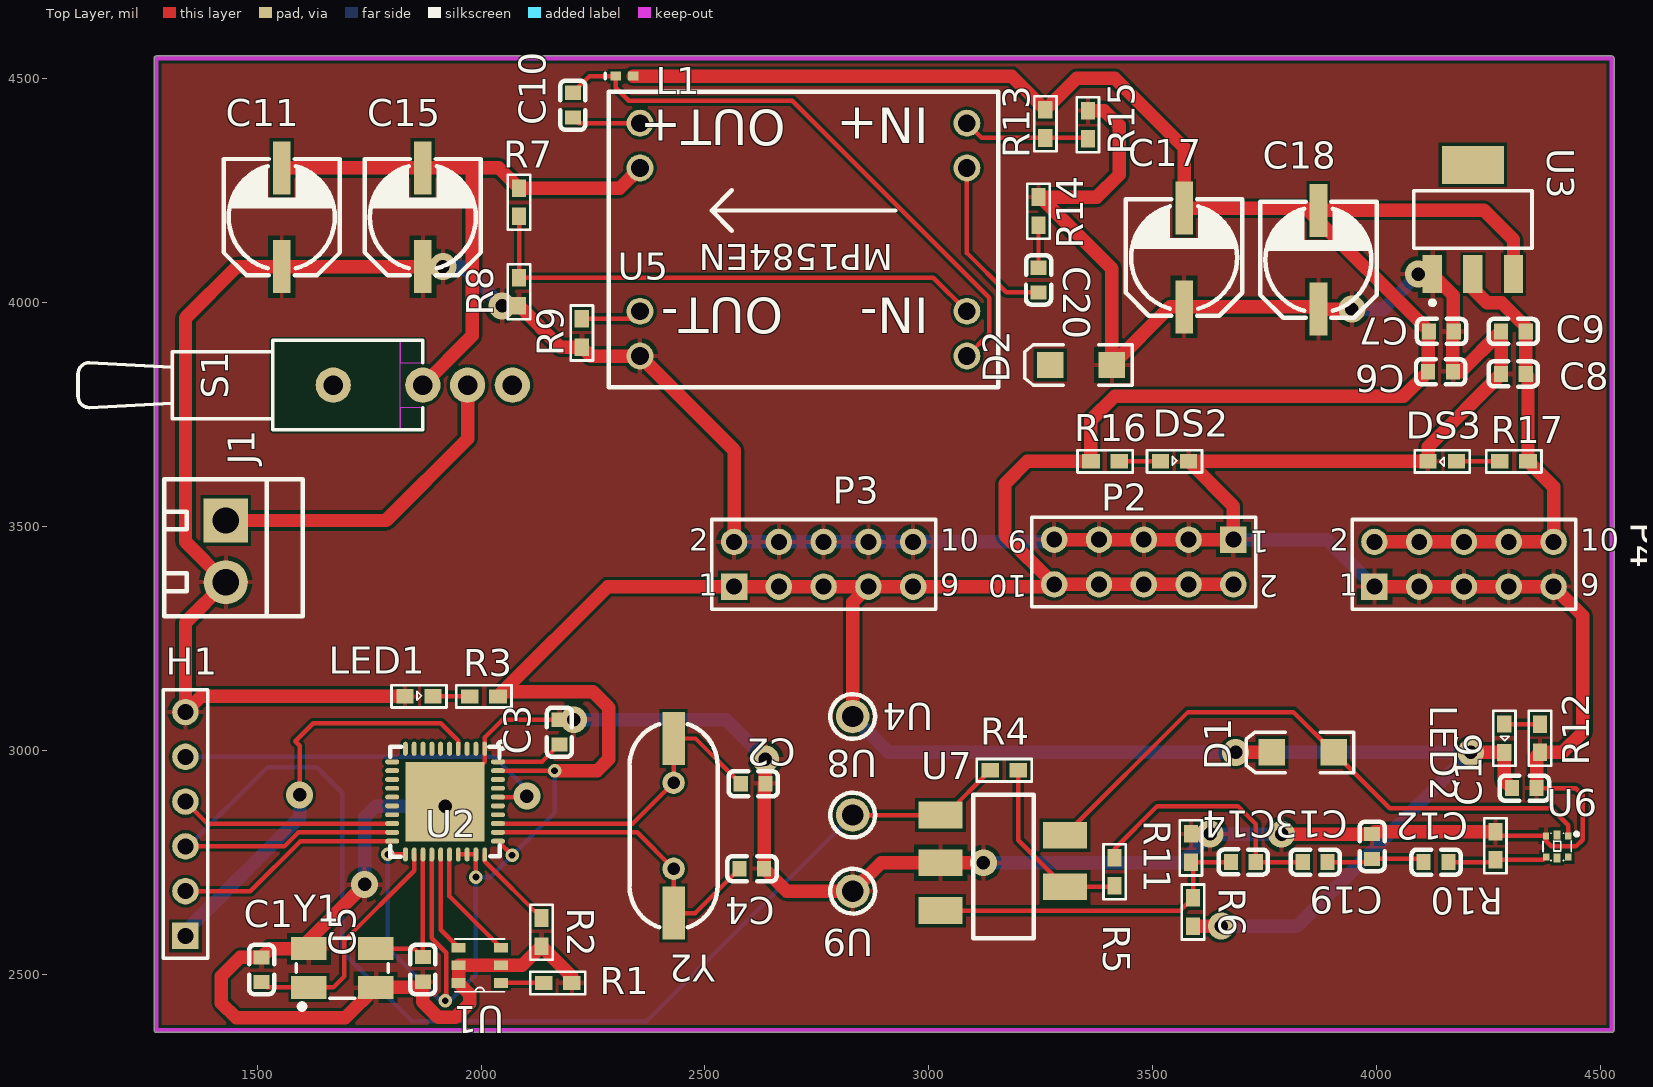
[diagram p0: Top Layer view]
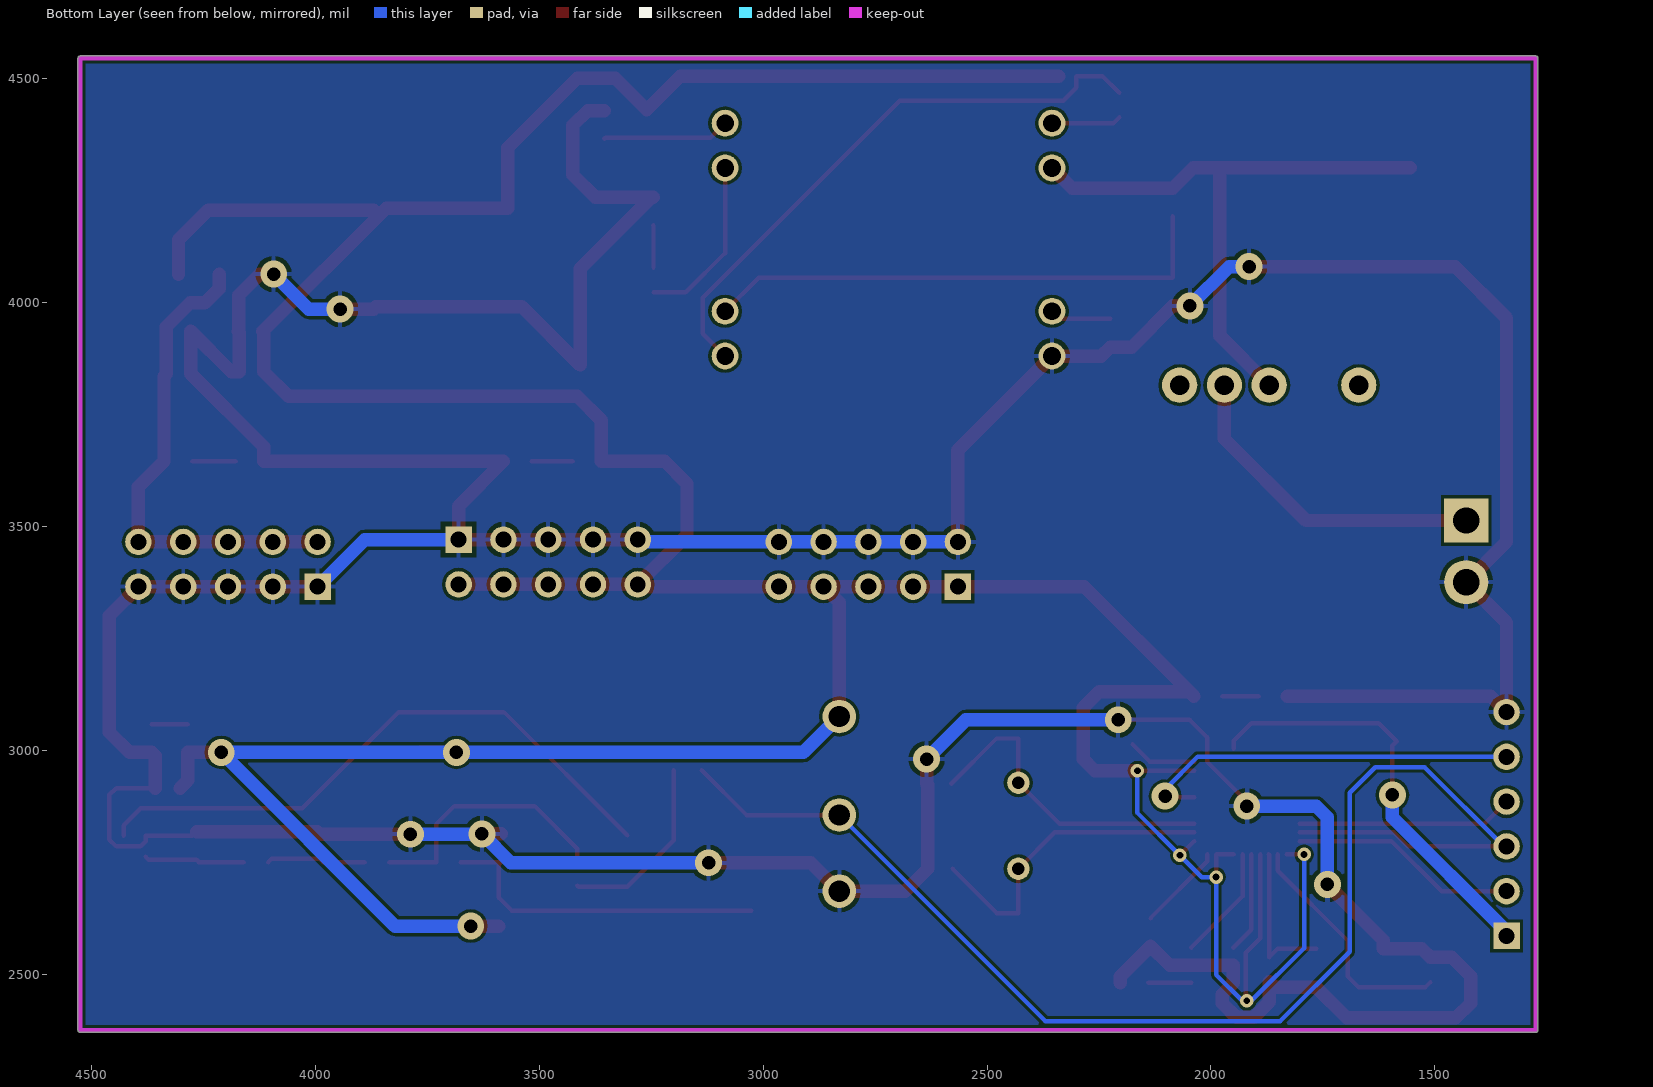
[diagram p1: Bottom Layer view, seen from below]
# Altium PCB MISC80555.PcbDoc
Units mil, origin at the board's own origin, x right, y up, seen from the top; angles counter-clockwise.
Board outline 3260.03 x 2180.03 mil, 2 copper layers (Top Layer, Bottom Layer); 61 components, 36 nets, 211 pads, 21 vias.

## Layer stack, top to bottom (the 12.6 mil dielectric is the usual default, probably not edited)
Top Solder: solder mask 0.4, Solder Resist, Dk 3.5
Top Layer: signal copper 1.4
Dielectric 1: dielectric 12.6, FR-4, Dk 4.8
Bottom Layer: signal copper 1.4
Bottom Solder: solder mask 0.4, Solder Resist, Dk 3.5

## Board outline
1275,2369.99 cw(c1275,2375) 1269.98,2375 1269.98,4545 cw(c1275,4545) 1275,4550.02 4525,4550.02 cw(c4525,4545) 4530.02,4545 4530.02,2375 cw(c4525,2375) 4525,2369.99

## Design rules (kind name [scope] priority, off if disabled: settings)
Clearance [All] p1: gap=7 ignorepadtopadclearanceinfootprint=FALSE except(0: Arc-Hole Track-Hole SMDPad-Hole THPad-Hole Via-Hole Fill-Hole Poly-Hole Region-Hole Text-Hole)
MinimumSolderMaskSliver [All] p1: minsoldermaskwidth=0
PolygonConnect [All] p1: connectstyle=Relief reliefconductorwidth=10 reliefentries=4 polygonreliefangle="90 Angle" airgapwidth=10
RoutingVias [All] p1: holewidth=28 width=50 viastyle="Through Hole" minholewidth=28 minwidth=50 maxholewidth=28 maxwidth=50
SilkToSilkClearance [All] p1: silktosilkclearance=0
SilkToSolderMaskClearance [IsPad] p1: minsilkscreentomaskgap=0 clearancetoexposedcopper=TRUE
SolderMaskExpansion [All] p1: expansion=4
Width [All] p1: maxlimit=30 minlimit=10 preferedwidth=10
27 further rules are at their usual default settings.

## Components (designator, comment, footprint, x,y, rotation, side; value= is the part's Value field where it differs from the comment)
C1 "100nF" C0603 1510,2510 r270 top
C2 "100nF" C0603 2607.75,2924.89 r180 top
C3 "100nF" C0603 2175,3040 r90 top
C4 "100nF" C0603 2605,2735 r180 top
C5 "100nF" C0603 1870,2510 r90 top
C6 "100nF" C0603 4142.86,3844.89 r180 top
C7 "100nF" C0603 4145,3935 r180 top
C8 "100nF" C0603 4305,3840 r0 top
C9 "100nF" C0603 4305,3935 r0 top
C10 "100nF" C0603 2205,4440 r90 top
C11 "220UF/25V" 贴片电容 1555,4190 r0 top
C12 "100nF" C0603 4132.75,2749.89 r180 top
C13 "100nF" C0603 3862.86,2749.89 r180 top
C14 "100nF" C0603 3702.25,2750.11 r0 top
C15 "10UF/50V" 贴片电容 1870,4190 r0 top
C16 "100nF" C0603 4330,2915 r180 top
C17 "22UF/50V" 贴片电容 3570,4100 r0 top
C18 "220UF/25V" 贴片电容 3870,4095 r0 top
C19 "100nF" C0603 3990,2785 r270 top
C20 "100nF" C0603 3245,4050 r270 top
D1 "D_1N4007A" 3.2X1.6X1.1 3835,2995 r180 top
D2 "Diode BAS16" 3.2X1.6X1.1 3340,3860 r180 top
DS2 "LED2" my0603LED 3517.01,3645 r0 top
DS3 "LED2" my0603LED 4177.99,3645 r180 top
H1 "HDR-F_2.54_1x6P" HDR1X6 1340,2585 r90 top
J1 "KF350-2P" KF350-2P 1430,3512.8 r270 top
L1 "10UH" 0402-A 2320.31,4505 r0 top
LED1 "LED_0603-R" my0603LED 1830,3120.24 r0 top
LED2 "LED_0603-R" my0603LED 4285,3057.99 r270 top
P2 "Header 5X2" HDR2X5 3680,3470 r180 top
P3 "Header 5X2" HDR2X5 2565,3365 r0 top
P4 "Header 5X2" HDR2X5 3995,3365 r0 top
R1 "10K" my0603 2140,2480 r0 top
R2 "10K" my0603 2135,2625 r270 top
R3 "10K" my0603 2037.99,3120 r180 top
R4 "10K" my0603 3137.01,2955 r0 top
R5 "10K" my0603 3415,2760 r270 top
R6 "10K" my0603 3590,2670 r270 top
R7 "10K" my0603 2085,4192.01 r90 top
R8 "10K" my0603 2085,3992.01 r90 top
R9 "10K" my0603 2225,3900 r90 top
R10 "10K" my0603 4265,2817.99 r270 top
R11 "10K" my0603 3585,2812.99 r270 top
R12 "10K" my0603 4365,2995 r90 top
R13 "10K" my0603 3260,4430 r270 top
R14 "10K" my0603 3245,4172.01 r90 top
R15 "10K" my0603 3355,4365 r90 top
R16 "10K" my0603 3425,3645 r180 top
R17 "10K" my0603 4337.99,3645 r180 top
S1 "SW-SPDT" TL36WW15050 1870,3815 r180 top
U1 "BL1" "TSOP-6 - duplicate" 1997.24,2519.37 r180 top
U2 "CC2540" CC254X_QFN 1920,2885 r270 top
U3 "LM1117-3.3" LM1117-3.3 4205,4175 r270 top
U4 "RH-5000" TEST-TH_BD2.54-P1.4_RED 2830,3075 r180 top
U5 "MP1584EN" MP1548EN 2720,4140 r180 top
U6 "APDS" SENSORS-SMD_APDS-9008-020 4410,2785 r0 top
U7 "AMP" MCP6001 3165,2740 r0 top
U8 "RH-5000" TEST-TH_BD2.54-P1.4_RED 2830,2855 r180 top
U9 "RH-5000" TEST-TH_BD2.54-P1.4_RED 2830,2685 r180 top
Y1 "12MHz" OSC-SMD_4P-L5.0-W3.2-BL 1690.2,2502.82 r0 top
Y2 "8MHz" XTAL_US 2430,2927.13 r270 top

## Footprints (in the part's own frame and the unit in brackets; to place one, negate y for a bottom-side part, rotate by r counter-clockwise, add the part's x,y. Pads: shape width x height; smd on the part's side, far side on the other; paste and mask are expansions set on the pad)
3.2X1.6X1.1 [mm] "SMT LED; 2 Flat Leads"
  rect 1.5x1.5 smd: 1(-1.75,0) 2(1.75,0)
  silkscreen extent -2.9,-1.15 3.2,1.15
0402-A [mm] "Chip Inductor, Body 1.0x0.5mm, IPC High Density"
  rect 0.6x0.5 smd: 1(-0.5,0) 2(0.5,0)
  silkscreen extent -1.1,-0.15 -1.1,0.15, body extent -0.55,-0.3 0.55,0.3, height 0.55
C0603 [mm]
  rect 0.8x0.9 smd paste+0 mask+0.051: 1(-0.692,-0.003) 2(0.708,-0.003)
  silkscreen extent -1.4,-0.71 1.4,0.71
CC254X_QFN [mm]
  oval 0.8x0.28 smd paste+0 mask+0.051: 1(-2.998,2.242) 2(-2.998,1.742) 3(-2.998,1.242) 4(-2.998,0.742) 5(-2.998,0.242) 6(-2.998,-0.258) 7(-2.998,-0.758) 8(-2.998,-1.258) 9(-2.998,-1.758) 10(-2.998,-2.258) 21(2.996,-2.254) 22(2.998,-1.758) 23(2.998,-1.258) 24(2.998,-0.758) 25(2.998,-0.258) 26(2.998,0.242) 27(2.998,0.742) 28(2.998,1.242) 29(2.998,1.742) 30(2.998,2.242)
  oval 0.28x0.8 smd paste+0 mask+0.051: 11(-2.256,-3.007) 12(-1.756,-3.007) 13(-1.256,-3.007) 14(-0.756,-3.007) 15(-0.256,-3.007) 16(0.244,-3.007) 17(0.744,-3.007) 18(1.244,-3.007) 19(1.744,-3.007) 20(2.244,-3.007) 31(2.244,2.99) 32(1.744,2.99) 33(1.244,2.99) 34(0.744,2.99) 35(0.244,2.99) 36(-0.256,2.99) 37(-0.756,2.99) 38(-1.256,2.99) 39(-1.756,2.99) 40(-2.256,2.99)
  rect 4.5x4.5 smd paste+0 mask+0.051: 41(0,-0.008)
  silkscreen extent -3.4,-3.12 3.12,3.41
HDR1X6 [mm] "Connector; Header; 6 Position"
  rect 1.5x1.5 hole 0.9: 1(0,0)
  round 1.5 hole 0.9: 2(2.54,0) 3(5.08,0) 4(7.62,0) 5(10.16,0) 6(12.7,0)
  silkscreen extent -1.27,-1.27 13.97,1.27
HDR2X5 [mm] "Connector; Header; 5x2 Position"
  rect 1.5x1.5 hole 0.9: 1(0,0)
  round 1.5 hole 0.9: 2(0,2.54) 3(2.54,0) 4(2.54,2.54) 5(5.08,0) 6(5.08,2.54) 7(7.62,0) 8(7.62,2.54) 9(10.16,0) 10(10.16,2.54)
  silkscreen extent -1.27,-1.27 11.43,3.81
KF350-2P [mm] "可拼接端子/10A"
  rect 2.5x2.5 hole 1.5: 1(0,0)
  round 2.5 hole 1.5: 2(3.5,0)
  silkscreen extent -2.34,-3.48 5.44,4.37, body extent -2.15,-3.34 5.25,4.16, height 10
LM1117-3.3 [mm]
  rect 2.15x1.1 smd: 1(2.846,-2.046) 2(2.846,0.254) 3(2.846,2.554)
  rect 2.15x3.5 smd: 4(-3.354,0.254)
  silkscreen extent -1.88,-3.1 4.6,3.6
MCP6001 [mil]
  rect 98.42x60 smd paste+4 mask+4: 1(-138.75,115) 2(-138.75,8.33) 3(-138.75,-98.33) 4(138.75,-45) 5(138.75,70)
  silkscreen extent -66,-160 69,160
MP1548EN [mil]
  round 60 hole 39.37 paste+4 mask+4: 1(-365.04,260) 2(-365.04,160) 3(-365.04,-160) 4(-365.04,-260) 5(364.96,260) 6(364.96,160) 7(364.96,-160) 8(364.96,-260)
  silkscreen extent -435,-330 435,330
my0603 [mm]
  rect 1x0.8 smd: 1(0,0) 2(1.6,0)
  silkscreen extent -0.76,-0.64 2.36,0.64
my0603LED [mm]
  rect 0.965x0.8 smd: 1(0,0) 2(1.6,0)
  silkscreen extent -0.76,-0.64 2.36,0.64
OSC-SMD_4P-L5.0-W3.2-BL [mm]
  rect 2x1.3 smd paste+0 mask+0.102: 1(-1.9,-0.834) 2(1.9,-0.834) 3(1.9,1.366) 4(-1.9,1.366)
  silkscreen extent -2.6,-2.07 2.6,1.97
SENSORS-SMD_APDS-9008-020 [mm]
  rect 0.35x0.4 smd paste+0 mask+0.051: 1(0.45,0.596) 3(-0.8,0.596) 4(-0.799,-0.6) 6(0.451,-0.6)
  rect 0.4x0.5 smd paste+0 mask+0.051: 2(-0.173,0.65) 5(-0.173,-0.65)
  silkscreen extent -0.98,-0.8 1.03,0.8
TEST-TH_BD2.54-P1.4_RED [mm]
  round 1.9 hole 1.2 paste+0 mask+0.051: 1(0,0)
  silkscreen extent -1.27,-1.27 1.27,1.27
TL36WW15050 [mm] "Switch; 4 Leads"
  round 2 hole 1.1: 1(0,0) 2(-2.54,0) 3(-5.08,0) M(5.08,0)
  Top Layer keep-out region: 1.27,2.54 1.27,-2.54 8.509,-2.54 8.509,2.54
  Top Layer keep-out region: 0,2.54 0,1.27 1.27,1.27 1.27,2.54
  Top Layer keep-out region: 0,-1.27 0,-2.54 1.27,-2.54 1.27,-1.27
  silkscreen extent 0,-2.54 19.56,2.54
"TSOP-6 - duplicate" [mm]
  rect 0.8x0.55 smd paste+0 mask+0.051: 1(-1.2,1) 2(-1.2,0) 3(-1.2,-1) 4(1.2,-1) 5(1.2,0) 6(1.2,1)
  silkscreen extent -1.4,-1.5 1.4,1.5
XTAL_US [mm]
  rect 3x1.27 smd: 1(-2.51,0) 2(7.39,0)
  round 1.27 hole 0.711: 1(0,0) 2(4.88,0)
  silkscreen extent -3.33,-2.5 8.21,2.5
贴片电容 [mm]
  rect 1x3 smd paste+0 mask+0.102: 1(0,-2.8) 2(0,2.8)
  silkscreen extent -3.3,-3.3 3.3,3.3

## Part data
C1 C2 C3 C4 C5 C6 C7 C8 C9 C10 C12 C13 C14 C16 C19 C20: library part CAP_0603
C11 C15 C17 C18: library part "Cap Semi", "Capacitor (Semiconductor SIM Model)"
D2: "Silicon Switching Diode for High-Speed Switching"
DS2 DS3: "Typical RED, GREEN, YELLOW, AMBER GaAs LED"
L1: library part Inductor, "Inductor"
P2 P3 P4: "Header, 5-Pin, Dual row"
R1 R2 R3 R4 R5 R6 R7 R8 R9 R10 R11 R12 R13 R14 R15 R16 R17: library part Res_0603
S1: "SPDT Subminiature Toggle Switch, Right Angle Mounting, Vertical Actuation"
U3: library part LM1117, "LINER REG"
Y1: library part X322512MSB4SI, "Crystal type: SMD crystal; frequency: 12MHz; frequency tolerance (room temp): ±10ppm; load capacitance: 20pF; frequency stability (full temp): ±20ppm;"
Y2: library part X49SM8MSD2SC, "Crystal type: SMD crystal; frequency: 8MHz; frequency tolerance (room temp): ±20ppm; load capacitance: 20pF; frequency stability (full temp): ±30ppm;"

## Via types
v1: diameter 60, hole 30, Top Layer to Bottom Layer, 16 vias
v2: diameter 30, hole 15, Top Layer to Bottom Layer, 5 vias

## Nets (pads, with @x,y where several pads share a name; then routed paths per layer and width w, separated by ;. In a path a pad name is that pad's centre, name@x,y a point inside that pad or via, vN(x,y) a via of type N, cw(c..) or ccw(c..) an arc to the next point about the centre after c; other vN are vias at no path point)
3V3: C8.2 C9.2 P4.2 P4.4 P4.6 P4.8 P4.10 R17.1 U3.2 | length 1091.8
  Top Layer w30: P4.2 P4.4 P4.6 P4.8 P4.10 4395,3587.99 R17.1 4337.99,3834.77 C8.2 C9.2 4332.86,3945.09 4279.32,3998.63 4246.37,3998.63 4215,4030 U3.2
ADC1: H1.3 R4.1 U2.19 U7.1 U8.1 | length 3019.7
  Top Layer w10: H1.3 1560.96,2785 1592.31,2816.35 U2.19 ; U8.1 U7.1 3037.01,2855 R4.1
  Bottom Layer w10: H1.3 1346,2785 1523,2962 1633,2962 1690,2905 1690,2550 1845,2395 2370,2395 U8.1
ADC2: H1.4 U2.18 | length 481.9
  Top Layer w10: H1.4 1388.96,2836.04 U2.18
EN: H1.5 U2.36 | length 873.2
  Top Layer w10: U2.36 2037.81,2895 2100,2895 v1(2102.27,2897.27)
  Bottom Layer w10: H1.5 2030,2985 2102.27,2912.73 v1(2102.27,2897.27)
GND: C1.1 C2.1 C3.2 C4.1 C5.1 C6.1 C7.1 C8.1 C9.1 C11.1 C15.1 C16.1 C17.1 C18.1 C19.1 D2.1 DS2.2 DS3.2 H1.6 J1.2 LED1.1 P2.1 P2.3 P2.5 P2.7 P2.9 P3.2 P3.4 P3.6 P3.8 P3.10 P4.1 P4.3 P4.5 P4.7 P4.9 R1.2 R2.2 R8.1 R9.1 R10.1 R11.1 R12.1 R14.2 R15.2 U1.2 U1.5 U1.6 U2.1 U2.41 U3.1 U5.5 U6.3 U7.2 U9.1 Y1.2 Y1.4 | length 13849.8
  Top Layer w10: U2.41 2008.25,2973.58 U2.1 2008.25,3028.25 2047.86,3067.86 C3.2 v1(2207.14,3067.86) ; R10.1 4274.54,2808.45 U6.3 4378.49,2796.51 4390,2785 4445,2785 4460,2800 4460,2900 4444.89,2915.11 C16.1
  Top Layer w30: v1(1740,2700) 1615.39,2575.39 Y1.4 1529.26,2556.61 C1.1 1462.25,2537.25 1420,2495 1420,2435 1453,2402 1697,2402 Y1.2 1857.35,2470 C5.1 1870.11,2437.57 1904.67,2403 1943,2403 1975,2435 1975,2455 U1.6 U1.5 U1.2 2092.36,2519.37 R2.2 2202.99,2494.02 R1.2 ; LED1.1 1375.24,3120.24 H1.6 1340,3285 J1.2 1340,3465 1340,3965 1454.76,4079.76 C11.1 C15.1 v1(1914.76,4079.76) ; v1(2047.01,3992.01) R8.1 2177.01,3900 R9.1 2245,3880 U5.5 2565,3670.04 P3.2 ; v1(2635,2980) C2.1 2632.25,2922.25 C4.1 2682.35,2685 U9.1 2893.33,2748.33 U7.2 v1(3121.67,2748.33) ; R14.2 R14.2@3248.55,4235 ; P2.9 P2.7 P2.5 P2.3 P2.1 3680,3545 DS2.2 DS3.2 4115,3677.14 C8.1 C9.1 4187.86,3845 C6.1 4170.11,3932.97 C7.1 4171.35,3936.01 4171.35,4016.05 U3.1 v1(4092.95,4062.95) ; R15.2 3392.01,4427.99 3425,4395 3425,4285 3375,4235 R14.2@3248.55,4235 ; R11.1 v1(3627.99,2812.99) ; v1(3787.75,2812.25) C19.1 3995.64,2817.99 R10.1 ; v1(3944.76,3984.76) C18.1 3865,3989.76 C17.1 3538.66,3989.76 D2.1 3408.9,4074.66 R14.2@3248.55,4235 ; P4.1 P4.3 P4.5 P4.7 P4.9 4460,3300 4460,3040 4415,2995 R12.1 4357.25,2987.25 C16.1
  Bottom Layer w30: v1(1740,2700) 1740,2850 1765,2875 v1(1920,2875) ; v1(1914.76,4079.76) 1959.25,4079.76 v1(2047.01,3992.01) ; v1(2207.14,3067.86) 2547.14,3067.86 v1(2635,2980) ; P3.2 P3.4 P3.6 P3.8 P3.10 3275,3465 P2.9 ; v1(3121.67,2748.33) 3563.33,2748.33 v1(3627.99,2812.99) 3628.74,2812.25 v1(3787.75,2812.25) ; P2.1 3890,3470 P4.1 ; v1(3944.76,3984.76) 4014.76,3984.76 v1(4092.95,4062.95)
NetC3_1: C3.1 U2.40 | length 153.5
  Top Layer w10: U2.40 2136.18,2973.83 C3.1
NetC10_1: C10.1 U5.8 | length 155.2
  Top Layer w10: C10.1 2217.86,4400 U5.8
NetC10_2: C10.2 L1.1 U5.1 | length 1316
  Top Layer w10: C10.2 2242.24,4505 L1.1 2300.63,4479.37 2330,4450 2695,4450 3135,4010 3135,3929.96 U5.1
NetC12_1: C12.1 R10.2 U6.4 | length 223.3
  Top Layer w10: C12.1 4260,2750 R10.2 4372.17,2755 U6.4
NetC12_2: C12.2 C13.1 C19.2 | length 220.7
  Top Layer w10: C13.1 3982.76,2750 C19.2 4097.75,2757.14 C12.2
NetC13_2: C13.2 C14.2 R5.1 | length 580.9
  Top Layer w10: R5.1 3415,2780 3510,2875 3690,2875 3730.11,2834.89 C14.2 C13.2
NetC14_1: C14.1 R6.1 R11.2 U7.3 | length 747.6
  Top Layer w10: U7.3 3561.67,2641.67 R6.1 3590,2745 R11.2 C14.1
NetC20_1: C20.1 R14.1 | length 94.8
  Top Layer w10: C20.1 3244.89,4171.9 R14.1
NetC20_2: C20.2 U5.3 | length 386.3
  Top Layer w10: U5.3 3085.04,4109.96 3172.86,4022.14 C20.2
NetD1_1: D1.1 U6.1 U7.5 | length 1366.4
  Top Layer w10: U7.5 3578.75,3085 3813.9,3085 D1.1 4028.9,2870 4390,2870 4427.7,2832.3 U6.1
NetDS2_1: DS2.1 R16.1 | length 92
  Top Layer w10: R16.1 DS2.1
NetDS3_1: DS3.1 R17.2 | length 97
  Top Layer w10: DS3.1 R17.2
NetJ1_1: J1.1 S1.2 | length 770.8
  Top Layer w10: S1.2@1945,3790 S1.2
  Top Layer w30: J1.1 1787.8,3512.8 1970,3695 S1.2
NetLED1_2: LED1.2 R3.2 | length 82.1
  Top Layer w10: LED1.2 1974.76,3120.24 R3.2
NetLED2_1: LED2.1 R12.2 | length 80
  Top Layer w10: LED2.1 R12.2
NetR1_1: R1.1 U1.1 | length 95.5
  Top Layer w10: U1.1 R1.1
NetR2_1: R2.1 U2.30 | length 194.5
  Top Layer w10: U2.30 2008.25,2751.75 R2.1
NetR4_2: R4.2 R5.2 U7.4 | length 415.1
  Top Layer w10: R4.2 3200,2798.75 U7.4 3412.99,2695 R5.2
NetR7_1: R7.1 R8.2 U5.2 | length 1168.1
  Top Layer w10: R7.1 R8.2 3010.04,4055 U5.2
NetR9_2: R9.2 U5.6 | length 137.1
  Top Layer w10: R9.2 2338.03,3962.99 U5.6
NetR13_2: R13.2 R15.1 U5.4 | length 284.5
  Top Layer w10: U5.4 3118.03,4367.01 R13.2 3352.99,4367.01 R15.1
NetU1_3: U1.3 U2.26 | length 255.8
  Top Layer w10: U2.26 1929.51,2673.71 U1.3
NetU1_4: U1.4 U2.25 | length 224.8
  Top Layer w10: U2.25 1909.83,2598.91 U1.4
POWER: H1.1 U2.4 | length 959.5
  Top Layer w10: v1(1595,2900) 1595,3010 1585,3020 1625,3060 1910,3060 1949.2,3020.8 U2.4
  Bottom Layer w30: H1.1 1340,2595 1595,2850 v1(1595,2900)
RES: H1.2 U2.20 | length 507.9
  Top Layer w10: H1.2 1485,2685 1596.67,2796.67 U2.20
VCC: C6.2 C7.2 C16.2 C17.2 C18.2 D1.2 L1.2 LED2.2 P2.2 P2.4 P2.6 P2.8 P2.10 P3.1 P3.3 P3.5 P3.7 P3.9 R3.1 R6.2 R13.1 R16.2 U2.21 U2.24 U2.27 U2.28 U2.29 U2.31 U2.39 U3.3 U4.1 | length 10807.2
  Top Layer w10: v2(1792.05,2767.05) U2.21 ; U2.24 1890.14,2579.86 1922.25,2547.75 1922.25,2453.71 1920,2453.71 v2(1920,2440) ; U2.27 U2.28 U2.29 v2(1988.57,2716.43) ; U2.31 v2(2069.39,2765) ; U2.39 v2(2164.15,2954.15)
  Top Layer w30: R3.1 R3.1@2047.99,3130 ; v2(2164.15,2954.15) 2259.15,2954.15 2285,2980 2285,3095 2250,3130 R3.1@2047.99,3130 ; L1.2 3185,4505 R13.1 3330,4500 3415,4500 3570,4345 C17.2 3842.01,4210.24 C7.2 4115,3932.97 C6.2 4060,3790 3415,3790 3362.01,3737.01 R16.2 3220,3645 3170,3595 3170,3480 P2.10 ; U4.1 2830,3330 P3.7 ; R6.2 v1(3652.99,2607.01) ; P2.2 P2.4 P2.6 P2.8 P2.10 ; v1(3685,2995) D1.2 ; C18.2 4239.76,4205.24 4305.55,4139.45 U3.3 ; v1(4210,2995) LED2.2 4285,2932.24 C16.2 ; R3.1@2047.99,3130 2282.99,3365 P3.1 P3.3 P3.5 P3.7 ; P3.7 P3.9 3275,3365 P2.10
  Bottom Layer w10: v2(1792.05,2767.05) 1792.05,2557.95 1910,2440 v2(1920,2440) 1930,2440 1988.57,2498.57 v2(1988.57,2716.43) 2020.82,2716.43 v2(2069.39,2765) 2164.15,2859.76 v2(2164.15,2954.15)
  Bottom Layer w30: U4.1 2910,2995 v1(3685,2995) v1(4210,2995) 3822.01,2607.01 v1(3652.99,2607.01)
VM: C11.2 C15.2 R7.2 S1.1 U5.7 | length 1368.2
  Top Layer w30: C11.2 C15.2 1980,4300.24 ; S1.1 1980,3925 1980,4300.24 ; U5.7 2310.04,4255 R7.2 2039.76,4300.24 1980,4300.24
X3: C2.2 U2.33 Y2.1 | length 720.5
  Top Layer w10: U2.33 2338.91,2836.04 2430,2927.13 2430,3025.94 2478.95,3025.94 C2.2
X4: C4.2 U2.32 Y2.2 | length 712.9
  Top Layer w10: U2.32 2348.65,2816.35 2430,2735 2430,2636.18 2478.21,2636.18 C4.2
Y1: C1.2 U2.22 Y1.1 | length 537
  Top Layer w10: C1.2 1522.03,2470 Y1.1 1670,2470 1695,2495 1695,2575 1850.77,2730.77 U2.22
Y2: C5.2 U2.23 Y1.3 | length 342.1
  Top Layer w10: Y1.3 1851.36,2556.61 C5.2 1870.11,2766.6 U2.23
pads on no net: D2.2 S1.3 S1.M U2.2 U2.3 U2.5 U2.6 U2.7 U2.8 U2.9 U2.10 U2.11 U2.12 U2.13 U2.14 U2.15 U2.16 U2.17 U2.34 U2.35 U2.37 U2.38 U3.4 U6.2 U6.5 U6.6

## Polygon pours and split planes (outlines as drawn)
GND on Top Layer "Top Layer-No Net" (solid, remove dead copper, pour order 4): 910,4800 1030,4680 4790,4680 4790,1950 4750,1910 4640,2020 840,2020
GND on Bottom Layer "Top Layer-No Net" (solid, remove dead copper, pour order 6): 870,4810 4780,4810 4880,4710 4825,4655 4825,2080 1085,2080 1010,2005

## Keep-outs
Keep-Out Layer:
  lines w10: 1375,4545 4525,4545 4525,2375 1275,2375 1275,4545 1425,4545